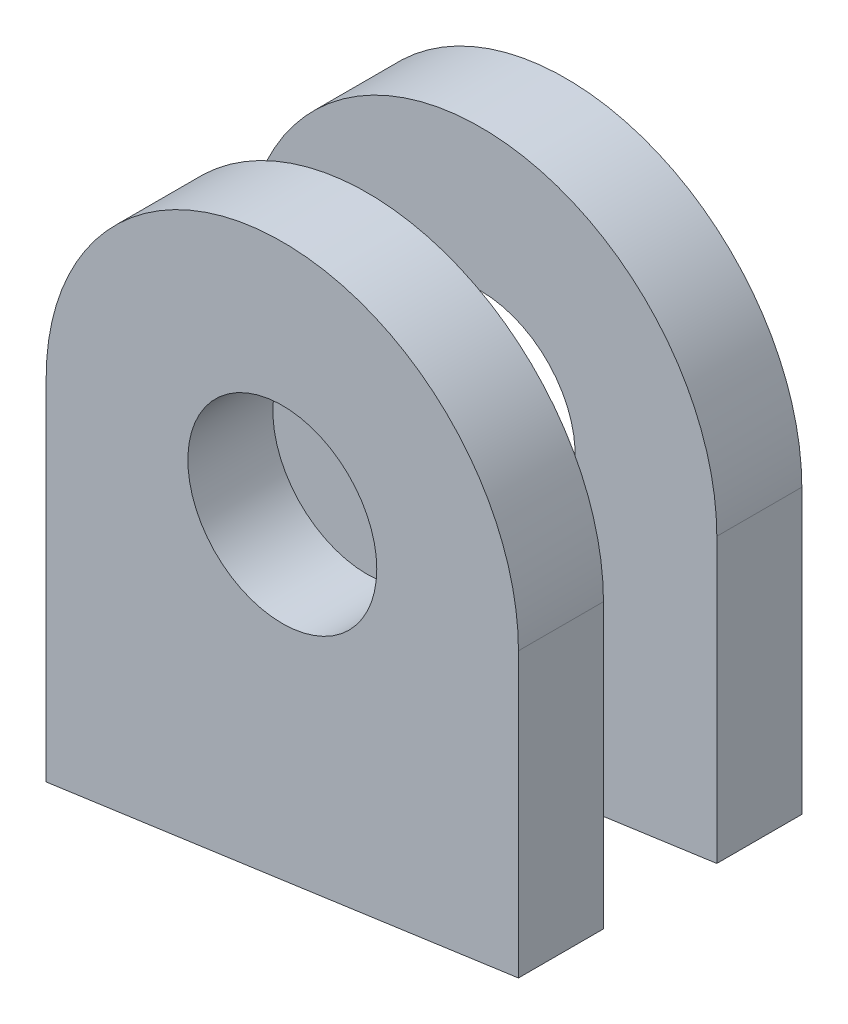
SolidWorks part; units mm, degrees
material "AISI 304"
ref_plane "Front Plane" through (0, 0, 0) normal (0, 0, 1) x (1, 0, 0)
ref_plane "Top Plane" through (0, 0, 0) normal (0, 1, 0) x (1, 0, 0)
ref_plane "Right Plane" through (0, 0, 0) normal (1, 0, 0) x (0, 0, -1)
other "Configuration Table"
sketch "Sketch1" plane through (0, 0, 0) normal (0, 0, 1) x (1, 0, 0)
  line L0 (-12.5, 0) -> (-12.5, -18.5135)
  line L1 (12.5, 0) -> (12.5, -15)
  line L2 (12.5, -15) -> (-12.5, -18.5135)
  circle A0 centre (0, 0) radius 5
  circle A1 centre (0, 0) radius 12.5
  dimension "D1" = 10
  dimension "D2" = 25
  dimension "D3" = 15
  dimension "D4" = 82
extrude "Boss-Extrude1" add sketch "Sketch1" along normal blind 15 contours A1 A0 | A1 L0 L2 L1
sketch "Sketch2" plane through (12.5, 0, 0) normal (1, 0, 0) x (0, 0, -1)
  line L0 (-15, 0) -> (0, 0) construction
  line L1 (-10.5, 57.4914) -> (-4.5, 57.4914)
  line L2 (-10.5, 57.4914) -> (-10.5, -57.4914)
  line L3 (-10.5, -57.4914) -> (-4.5, -57.4914)
  line L4 (-4.5, 57.4914) -> (-4.5, -57.4914)
  line L5 (-10.5, 57.4914) -> (-4.5, -57.4914) construction
  line L6 (-10.5, -57.4914) -> (-4.5, 57.4914) construction
  point P0 (-7.5, 0)
  dimension "D1" = 6
extrude "Cut-Extrude1" cut sketch "Sketch2" against normal through all both and the other way through all
